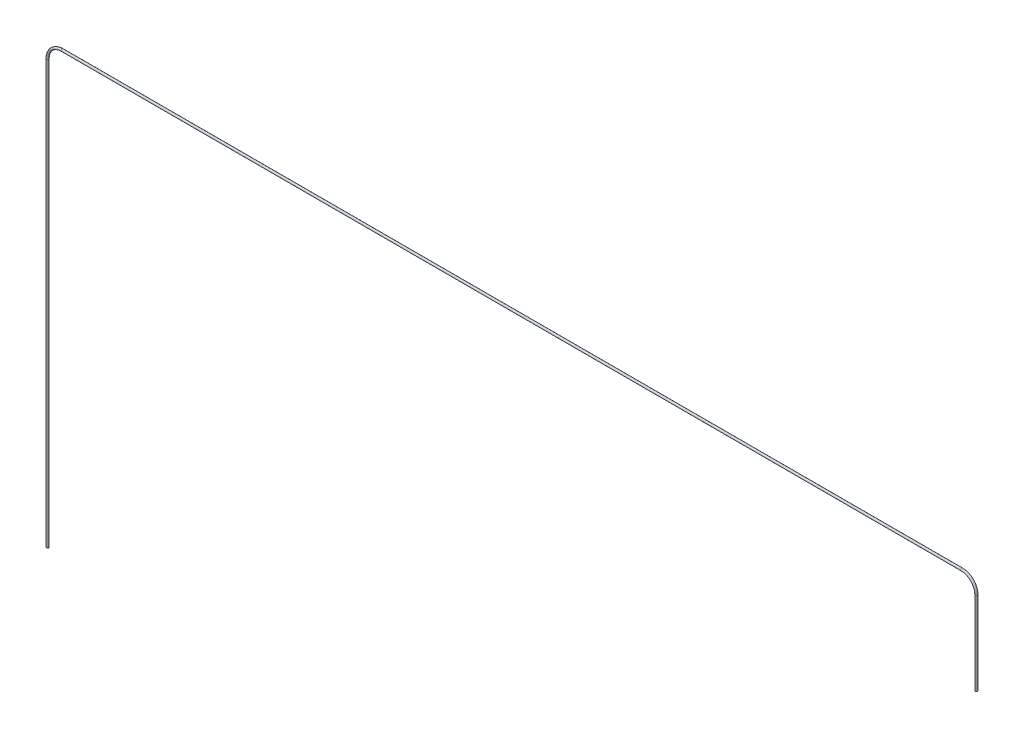
from build123d import *

# Parameters (mm, degrees)
SKETCH2_R = 3.25


with BuildPart() as part:
    # Sweep1: sweep along a path in Sketch1
    with BuildLine(Plane.XY) as sweep1_path:
        Line((0, 0), (0, 1213))
        ThreePointArc((0, 1213), (12.30151519, 1242.69848481), (42, 1255))
        Line((42, 1255), (2620, 1255))
        ThreePointArc((2620, 1255), (2649.69848481, 1242.69848481), (2662, 1213))
        Line((2662, 1213), (2662, 975))
    # Sketch2 → Sweep1 (sweep)
    with BuildSketch(Plane(origin=(0, 0, 0), x_dir=(1, 0, 0), z_dir=(0, 1, 0))):
        Circle(SKETCH2_R)
    sweep(path=sweep1_path.line)


solid = part.part
